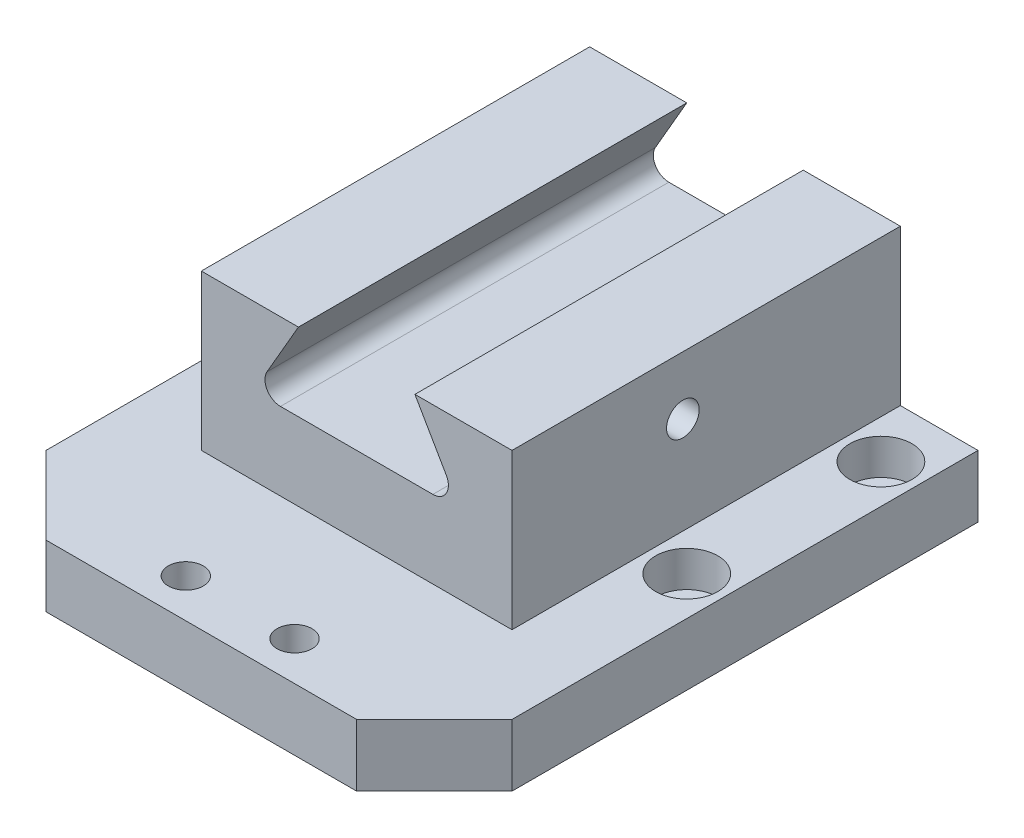
from build123d import *

# Parameters (mm, degrees)
SKETCH1_W                                            = 40
SKETCH1_H                                            = 20
BOSS_EXTRUDE1_DEPTH                                  = 25
SKETCH2_W                                            = 60
SKETCH2_H                                            = 70
BOSS_EXTRUDE2_DEPTH                                  = 8
CUT_EXTRUDE1_DEPTH                                   = 62.02458521
CHAMFER1_SIZE                                        = 10
HOLE_SIZE_PER_SOCKET_HEAD_CAP_SCREW_TYPE_D           = 4.5
HOLE_SIZE_PER_SOCKET_HEAD_CAP_SCREW_TYPE_CBORE_D     = 8
HOLE_SIZE_PER_SOCKET_HEAD_CAP_SCREW_TYPE_CBORE_DEPTH = 4.6
HOLE_SIZE_PER_SOCKET_HEAD_CAP_SCREW_2_D              = 4.5
HOLE_SIZE_PER_SOCKET_HEAD_CAP_SCREW_2_CBORE_D        = 8
HOLE_SIZE_PER_SOCKET_HEAD_CAP_SCREW_2_CBORE_DEPTH    = 4.6
M5_TAPPED_HOLE1_D                                    = 4.2
M5_TAPPED_HOLE1_DEPTH                                = 12.4
M5_TAPPED_HOLE1_TIP                                  = 1.2618073
M3_TAPPED_HOLE1_D                                    = 2.5
M3_TAPPED_HOLE1_DEPTH                                = 7.5
M3_TAPPED_HOLE1_TIP                                  = 0.751075774


with BuildPart() as part:
    # Sketch1 → Boss-Extrude1 (new, symmetric)
    with BuildSketch(Plane.XY):
        Rectangle(SKETCH1_W, SKETCH1_H)
    extrude(amount=BOSS_EXTRUDE1_DEPTH, both=True)

    # Sketch2 → Boss-Extrude2 (add)
    with BuildSketch(Plane.XZ.offset(10)):
        with Locations((0, 10)):
            Rectangle(SKETCH2_W, SKETCH2_H)
    extrude(amount=BOSS_EXTRUDE2_DEPTH)

    # Sketch3 → Cut-Extrude1 (cut, through all)
    with BuildSketch(Plane.XY.offset(25)):
        with BuildLine():
            Line((-7.5, 10), (-11.541451884, 3))
            ThreePointArc((-11.541451884, 3), (-11.541451884, 1), (-9.809401077, 0))
            Line((-9.809401077, 0), (9.809401077, 0))
            ThreePointArc((9.809401077, 0), (11.541451884, 1), (11.541451884, 3))
            Line((11.541451884, 3), (7.5, 10))
            Line((7.5, 10), (-7.5, 10))
        make_face()
    extrude(amount=-CUT_EXTRUDE1_DEPTH, mode=Mode.SUBTRACT)

    # Chamfer1
    chamfer1_edges = [part.edges().sort_by_distance(p)[0] for p in [
        (-30, -14, 45),
        (30, -14, 45),
    ]]
    chamfer(chamfer1_edges, length=CHAMFER1_SIZE)

    # Hole Size per Socket Head Cap Screw Type (through all)
    with Locations(Plane.XZ.offset(18)):
        with Locations((7, 40), (-7, 40)):
            CounterBoreHole(HOLE_SIZE_PER_SOCKET_HEAD_CAP_SCREW_TYPE_D / 2, HOLE_SIZE_PER_SOCKET_HEAD_CAP_SCREW_TYPE_CBORE_D / 2, HOLE_SIZE_PER_SOCKET_HEAD_CAP_SCREW_TYPE_CBORE_DEPTH)

    # Hole Size per Socket Head Cap Screw  2 (through all)
    with Locations(Plane(origin=(0, -10, 0), x_dir=(-1, 0, 0), z_dir=(0, 1, 0))):
        with Locations((25, -17.5), (25, 7.5), (-25, -17.5), (-25, 7.5)):
            CounterBoreHole(HOLE_SIZE_PER_SOCKET_HEAD_CAP_SCREW_2_D / 2, HOLE_SIZE_PER_SOCKET_HEAD_CAP_SCREW_2_CBORE_D / 2, HOLE_SIZE_PER_SOCKET_HEAD_CAP_SCREW_2_CBORE_DEPTH)

    # M5 Tapped Hole1
    with Locations(Plane(origin=(20, 0, 0), x_dir=(0, 0, -1), z_dir=(1, 0, 0))):
        with Locations((-3, 2.5)):
            Hole(M5_TAPPED_HOLE1_D / 2, depth=M5_TAPPED_HOLE1_DEPTH)
            with Locations((0, 0, -(M5_TAPPED_HOLE1_DEPTH + M5_TAPPED_HOLE1_TIP / 2))):  # 118° drill point
                Cone(0, M5_TAPPED_HOLE1_D / 2, M5_TAPPED_HOLE1_TIP, mode=Mode.SUBTRACT)

    # M3 Tapped Hole1
    with Locations(Plane(origin=(0, 0, -25), x_dir=(-1, 0, 0), z_dir=(0, 0, -1))):
        with Locations((14, 5), (-14, 5)):
            Hole(M3_TAPPED_HOLE1_D / 2, depth=M3_TAPPED_HOLE1_DEPTH)
            with Locations((0, 0, -(M3_TAPPED_HOLE1_DEPTH + M3_TAPPED_HOLE1_TIP / 2))):  # 118° drill point
                Cone(0, M3_TAPPED_HOLE1_D / 2, M3_TAPPED_HOLE1_TIP, mode=Mode.SUBTRACT)


solid = part.part
